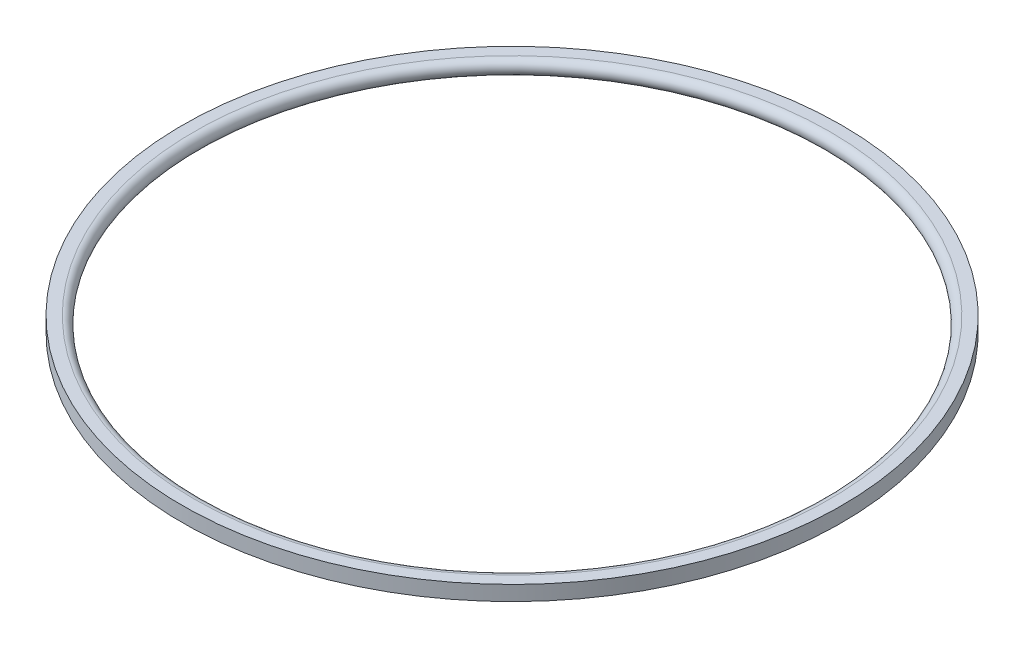
SolidWorks part; units mm, degrees
ref_plane "Front Plane" through (0, 0, 0) normal (0, 0, 1) x (1, 0, 0)
ref_plane "Top Plane" through (0, 0, 0) normal (0, 1, 0) x (1, 0, 0)
ref_plane "Right Plane" through (0, 0, 0) normal (1, 0, 0) x (0, 0, -1)
sketch "Sketch1" plane through (0, 0, 0) normal (0, 0, 1) x (1, 0, 0)
  line L0 (-171, 0) -> (-177.2, 0)
  line L1 (55, 0) -> (-55, 0) construction
  line L2 (-177.2, 0) -> (-177.2, 8)
  line L3 (-177.2, 8) -> (-171, 8)
  line L4 (0, 0) -> (0, 50000) construction
  line L5 (0, -55) -> (0, 55) construction
  arc A0 (-171, 0) -> (-171, 8) centre (-171, 4) ccw
  dimension "D3" = 171
  dimension "D4" = 4
  dimension "D1" = 8
  dimension "D2" = 177.2
revolve "Revolve1" add sketch "Sketch1" angle 360 about L4
